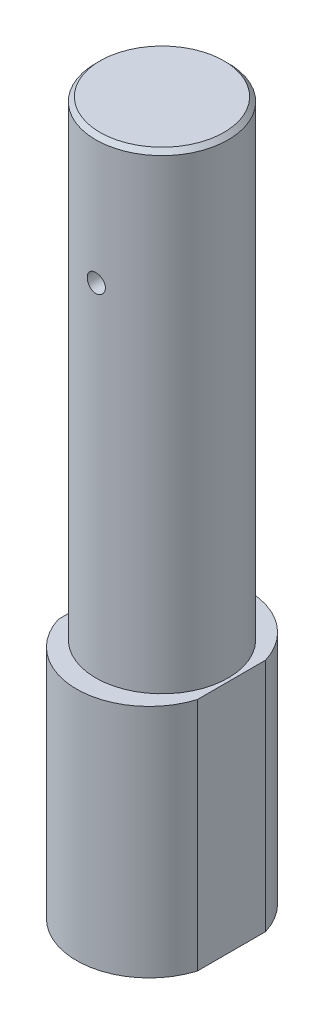
SolidWorks part; units mm, degrees
material "45"
ref_plane "前视基准面" through (0, 0, 0) normal (0, 0, 1) x (1, 0, 0)
ref_plane "上视基准面" through (0, 0, 0) normal (0, 1, 0) x (1, 0, 0)
ref_plane "右视基准面" through (0, 0, 0) normal (1, 0, 0) x (0, 0, -1)
sketch "草图1" plane through (0, 0, 0) normal (0, 1, 0) x (1, 0, 0)
  line L0 (0, 6) -> (0, -6) construction
  line L5 (0, 0) -> (32.5, 0) construction
  line L6 (32.5, -15.9875) -> (32.5, 15.9875)
  line L7 (-32.5, -15.9875) -> (-32.5, 15.9875)
  arc A0 (32.5, 15.9875) -> (-32.5, 15.9875) centre (0, 6) ccw
  arc A1 (32.5, -15.9875) -> (-32.5, -15.9875) centre (0, -6) cw
  point P4 (0, 40)
  point P11 (-32.5, 0)
  point P12 (0, -40)
  dimension "D1" = 68
  dimension "D2" = 32.5
  dimension "D3" = 6
  dimension "D4" = 80
extrude "凸台-拉伸1" add sketch "草图1" along normal blind 110
sketch "草图2" plane through (0, 110, 0) normal (0, 1, 0) x (1, 0, 0)
  circle A0 centre (0, 0) radius 31
  dimension "D1" = 62
extrude "凸台-拉伸2" add sketch "草图2" along normal blind 220
ref_plane "基准面1" through (0, 0, 31) normal (0, 0, 1) x (1, 0, 0)
hole_wizard "M10 螺纹孔1" positions "草图3" profile "草图4" tap size "M10" standard "GB"
sketch "草图3" plane through (0, 0, 31) normal (0, 0, 1) x (1, 0, 0)
  line L0 (32.5, 110) -> (-32.5, 110) construction
  point P0 (0, 270)
  dimension "D1" = 160
sketch "草图4" plane through (0, 270, 31) normal (1, 0, 0) x (0, -1, 0)
  line L0 (0, 0) -> (0, 30.0537)
  line L1 (0, 30.0537) -> (4.25, 27.5)
  line L2 (4.25, 27.5) -> (4.25, 0)
  line L5 (4.25, 0) -> (0, 0)
  line L10 (0, 30.0537) -> (-4.25, 27.5) construction
  line L11 (0, -6.35) -> (0, 107.95) construction
  dimension "螺纹孔钻头直径" = 8.5
  dimension "螺纹孔钻头深度" = 27.5
  dimension "导头角度" = 118
cosmetic thread "孔螺蚊线1" parameters "D1"=20, "D2"=10
chamfer "倒角1" distance 2 angle 45 1 edges at (0, 330, 31)
sketch "草图5" plane through (0, 0, 0) normal (0, 0, 1) x (1, 0, 0)
  line L0 (0, 23) -> (0, -33)
  arc A0 (0, -33) -> (0, 23) centre (0, -5) ccw
  dimension "D1" = 56
  dimension "D2" = 5
revolve "切除-旋转1" cut sketch "草图5" angle 360 about L0
